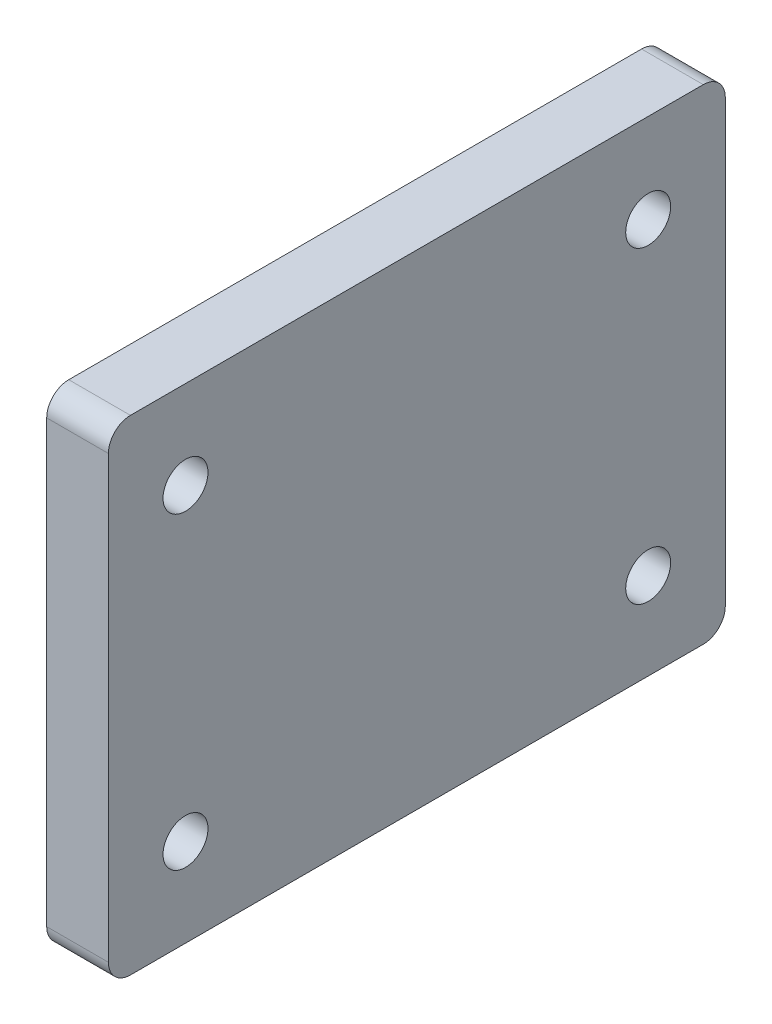
from build123d import *

# Parameters (mm, degrees)
SKETCH1_W                    = 140
SKETCH1_H                    = 110
BOSS_EXTRUDE1_DEPTH          = 14
FILLET1_R                    = 5
M12_TAPPED_HOLE1_D           = 10.2
M12_TAPPED_HOLE1_DEPTH       = 32.75
M12_TAPPED_HOLE1_CSINK_D     = 12.05
M12_TAPPED_HOLE1_CSINK_ANGLE = 90
M12_TAPPED_HOLE1_TIP         = 3.064389157


with BuildPart() as part:
    # Sketch1 → Boss-Extrude1 (new body)
    with BuildSketch(Plane(origin=(0, 0, 0), x_dir=(0, 0, -1), z_dir=(1, 0, 0))):
        Rectangle(SKETCH1_W, SKETCH1_H)
    extrude(amount=BOSS_EXTRUDE1_DEPTH)

    # Fillet1
    fillet1_edges = [part.edges().sort_by_distance(p)[0] for p in [
        (7, -55, -70),
        (7, -55, 70),
        (7, 55, 70),
        (7, 55, -70),
    ]]
    fillet(fillet1_edges, radius=FILLET1_R)

    # M12 Tapped Hole1
    with Locations(Plane.ZY):
        with Locations((-52.5, 34.756569307), (52.499717816, 35), (52.5, -35), (-52.5, -35.243430693)):
            CounterSinkHole(M12_TAPPED_HOLE1_D / 2, M12_TAPPED_HOLE1_CSINK_D / 2, depth=M12_TAPPED_HOLE1_DEPTH, counter_sink_angle=M12_TAPPED_HOLE1_CSINK_ANGLE)
            with Locations((0, 0, -(M12_TAPPED_HOLE1_DEPTH + M12_TAPPED_HOLE1_TIP / 2))):  # 118° drill point
                Cone(0, M12_TAPPED_HOLE1_D / 2, M12_TAPPED_HOLE1_TIP, mode=Mode.SUBTRACT)


solid = part.part
